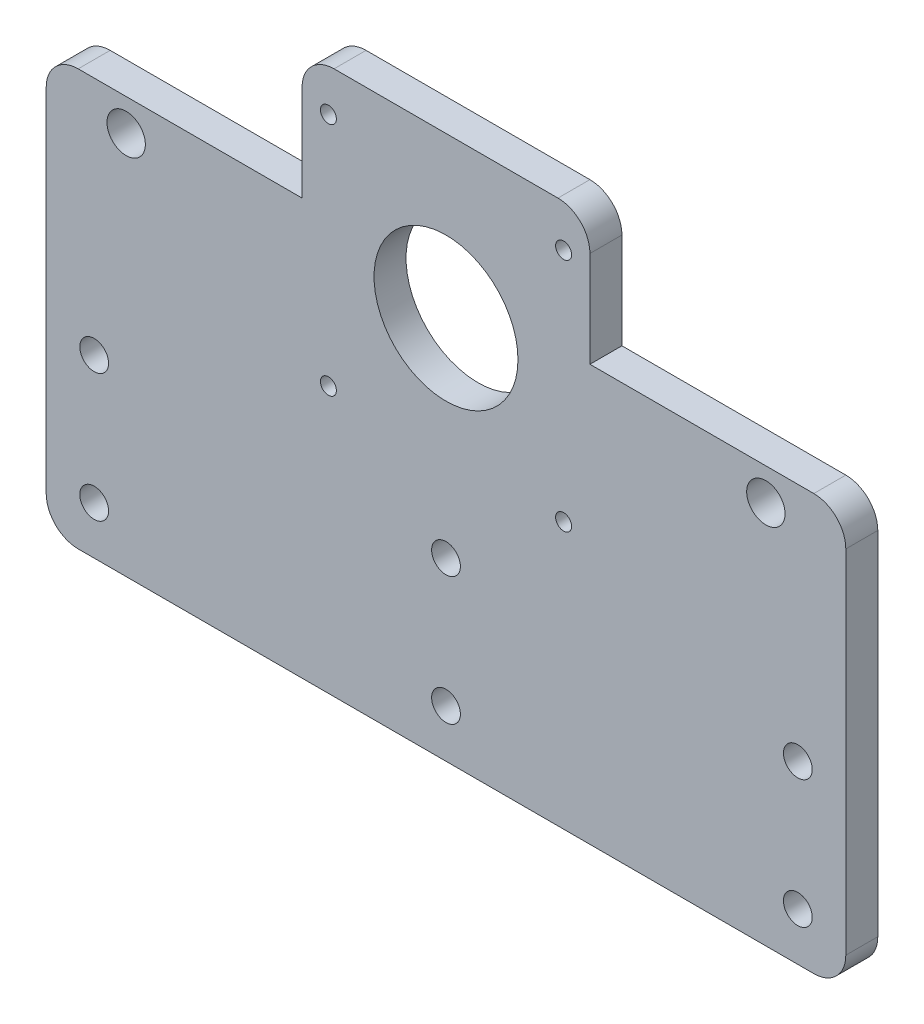
SolidWorks part; units mm, degrees
ref_plane "前视基准面" through (0, 0, 0) normal (0, 0, 1) x (1, 0, 0)
ref_plane "上视基准面" through (0, 0, 0) normal (0, 1, 0) x (1, 0, 0)
ref_plane "右视基准面" through (0, 0, 0) normal (1, 0, 0) x (0, 0, -1)
sketch "草图1" plane through (0, 0, 0) normal (0, 0, 1) x (1, 0, 0)
  line L1 (-125, 85) -> (125, 85)
  line L2 (-125, 85) -> (-125, -85)
  line L3 (-125, -85) -> (125, -85)
  line L4 (125, 85) -> (125, -85)
  line L5 (-125, 85) -> (125, -85) construction
  line L6 (-125, -85) -> (125, 85) construction
  point P0 (0, 0)
  dimension "D1" = 170
  dimension "D2" = 250
extrude "凸台-拉伸1" add sketch "草图1" along normal mid plane 10
sketch "草图2" plane through (0, 0, 5) normal (0, 0, 1) x (1, 0, 0)
  line L1 (125, 85) -> (45, 85)
  line L2 (125, 85) -> (125, 45)
  line L3 (125, 45) -> (45, 45)
  line L4 (45, 85) -> (45, 45)
  dimension "D1" = 80
  dimension "D2" = 40
extrude "切除-拉伸1" cut sketch "草图2" against normal blind 10
mirror "镜向1" about plane through (0, 0, 0) normal (1, 0, 0) of "切除-拉伸1"
hole_wizard "Ø9.0 (9) 直径孔1" positions "草图4" profile "草图3" hole size "Ø9.0" standard "GB" end condition up to next
sketch "草图4" plane through (0, 0, 5) normal (0, 0, 1) x (1, 0, 0)
  line L0 (-125, -85) -> (125, -85) construction
  line L1 (-125, 45) -> (-125, -85) construction
  point P0 (-110, -70)
  point P2 (-110, -30)
  dimension "D1" = 15
  dimension "D2" = 40
  dimension "D3" = 15
sketch "草图3" plane through (-110, -70, 5) normal (1, 0, 0) x (0, -1, 0)
  line L0 (0, 0) -> (0, 10)
  line L1 (0, 10) -> (4.5, 10)
  line L2 (4.5, 10) -> (4.5, 0)
  line L5 (4.5, 0) -> (0, 0)
  line L11 (0, -6.35) -> (0, 107.95) construction
  dimension "通孔孔直径" = 9
  dimension "通孔孔深度" = 10
pattern_linear "阵列(线性)1" count 3 spacing 110 along (1, 0, 0) of "Ø9.0 (9) 直径孔1"
hole_wizard "Ø12.0 (12) 直径孔1" positions "草图6" profile "草图5" hole size "Ø12.0" standard "GB" end condition up to next
sketch "草图6" plane through (0, 0, 5) normal (0, 0, 1) x (1, 0, 0)
  line L0 (-125, -85) -> (125, -85) construction
  point P0 (-100, 35)
  point P2 (100, 35)
  dimension "D1" = 120
  dimension "D2" = 200
  dimension "D3" = 100
sketch "草图5" plane through (-100, 35, 5) normal (1, 0, 0) x (0, -1, 0)
  line L0 (0, 0) -> (0, 10)
  line L1 (0, 10) -> (6, 10)
  line L2 (6, 10) -> (6, 0)
  line L5 (6, 0) -> (0, 0)
  line L11 (0, -6.35) -> (0, 107.95) construction
  dimension "通孔孔直径" = 12
  dimension "通孔孔深度" = 10
sketch "草图7" plane through (0, 0, 5) normal (0, 0, 1) x (1, 0, 0)
  line L0 (-125, -85) -> (125, -85) construction
  circle A0 centre (0, 35) radius 22.5
  dimension "D1" = 45
  dimension "D2" = 120
extrude "切除-拉伸2" cut sketch "草图7" against normal blind 10
hole_wizard "M6 螺纹孔1" positions "草图9" profile "草图8" tap size "M6" standard "ISO" end condition up to next
sketch "草图9" plane through (0, 0, 5) normal (0, 0, 1) x (1, 0, 0)
  circle A0 centre (0, 35) radius 22.5 construction
  point P10 (-36.77, 71.77)
  dimension "D1" = 36.77
  dimension "D2" = 36.77
sketch "草图8" plane through (-36.77, 71.77, 5) normal (1, 0, 0) x (0, -1, 0)
  line L0 (0, 0) -> (0, 10)
  line L1 (0, 10) -> (2.5, 10)
  line L2 (2.5, 10) -> (2.5, 0)
  line L5 (2.5, 0) -> (0, 0)
  line L11 (0, -6.35) -> (0, 107.95) construction
  dimension "通孔螺纹孔钻头直径" = 5
  dimension "通孔螺纹孔钻头深度" = 10
cosmetic thread "孔螺蚊线1" parameters "D2"=6
pattern_linear "阵列(线性)3" count 2 spacing 73.54 along (0, -1, 0) of "M6 螺纹孔1"
pattern_linear "阵列(线性)4" count 2 spacing 73.54 along (1, 0, 0) of "M6 螺纹孔1", "阵列(线性)3"
fillet "圆角1" radius 10 6 edges at (-125, -85, 0) (125, -85, 0) (125, 45, 0) (-125, 45, 0) (-45, 85, 0) (45, 85, 0)
